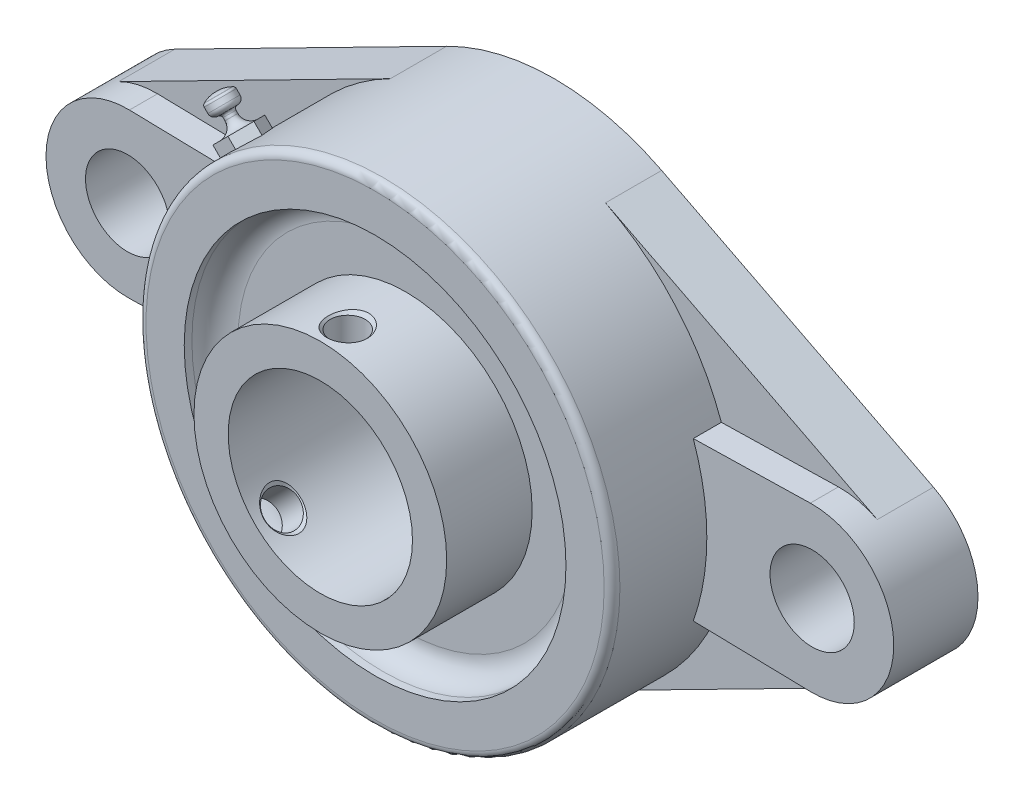
from build123d import *
from build123d.topology import SkipClean

# Parameters (mm, degrees)
SKETCH2_W          = 10.260420585
SKETCH2_H          = 10.310228453
CUT_EXTRUDE1_DEPTH = 4
SKETCH4_W          = 468
SKETCH4_H          = 360
CUT_EXTRUDE2_DEPTH = 44.4
SKETCH5_W          = 234
SKETCH5_H          = 180
CUT_EXTRUDE3_DEPTH = 5.333333333
SKETCH6_R          = 8
CUT_EXTRUDE4_DEPTH = 16
SKETCH7_R          = 8
CUT_EXTRUDE5_DEPTH = 16


with BuildPart() as part:
    # Sketch1 → Revolve1 (revolve)
    with BuildSketch(Plane(origin=(0, 0, 0), x_dir=(0, 0, -1), z_dir=(0.7071067811865476, 0.7071067811865475, 0)), mode=Mode.PRIVATE) as revolve1_sk:
        with BuildLine():
            Line((-4.44, 53), (-4.26179677, 53))
            ThreePointArc((-4.26179677, 53), (-3.226520589, 52.863703305), (-2.26179677, 52.464101615))
            Line((-2.26179677, 52.464101615), (-2.19, 52.422649731))
            ThreePointArc((-2.19, 52.422649731), (-2.006987298, 52.239637029), (-1.94, 51.989637029))
            Line((-1.94, 51.989637029), (-1.94, 51))
            ThreePointArc((-1.94, 51), (-2.232893219, 50.292893219), (-2.94, 50))
            ThreePointArc((-2.94, 50), (-3.293553391, 49.853553391), (-3.44, 49.5))
            Line((-3.44, 49.5), (-3.44, 49))
            ThreePointArc((-3.44, 49), (-2.854213562, 47.585786438), (-1.44, 47))
            Line((-1.44, 47), (0.56, 47))
            Line((0.56, 47), (0.56, 43))
            Line((0.56, 43), (-4.44, 43))
            Line((-4.44, 43), (-4.44, 53))
        make_face()
    revolve(revolve1_sk.sketch.rotate(Axis((-30.405591591, 30.405591591, 4.44), (-0.7071067811865477, 0.7071067811865474, 0)), 90), axis=Axis((-30.405591591, 30.405591591, 4.44), (-0.7071067811865477, 0.7071067811865474, 0)))

    # Sketch2 → Cut-Extrude1 (cut)
    with BuildSketch(Plane(origin=(-30.405591591, 30.405591591, 0), x_dir=(0, 0, -1), z_dir=(0.7071067811865501, -0.7071067811865449, 0))):
        with Locations((-4.564519667, -0.074711801)):
            Rectangle(SKETCH2_W, SKETCH2_H)
        Polygon((-7.94, 2.020725942), (-7.94, -2.020725942), (-4.44, -4.041451884), (-0.94, -2.020725942), (-0.94, 2.020725942), (-4.44, 4.041451884), align=None, mode=Mode.SUBTRACT)
    extrude(amount=-CUT_EXTRUDE1_DEPTH, mode=Mode.SUBTRACT)

    # Sketch3 → Revolve2 (revolve)
    with BuildSketch(Plane(origin=(0, 0, 0), x_dir=(0, 0, -1), z_dir=(1, 0, 0)), mode=Mode.PRIVATE) as revolve2_sk:
        with BuildLine():
            Line((-22.2, 24), (-22.2, 17.5))
            Line((-22.2, 17.5), (20.7, 17.5))
            Line((20.7, 17.5), (20.7, 24))
            Line((20.7, 24), (19.533333333, 24))
            ThreePointArc((19.533333333, 24), (15.408543776, 25.708543776), (13.7, 29.833333333))
            Line((13.7, 29.833333333), (13.7, 31.875))
            ThreePointArc((13.7, 31.875), (14.981407832, 34.968592168), (18.075, 36.25))
            Line((18.075, 36.25), (22.2, 36.25))
            Line((22.2, 36.25), (22.2, 80.5))
            Line((22.2, 80.5), (6.2, 80.5))
            Line((6.2, 80.5), (6.2, 45))
            Line((6.2, 45), (-10.3, 45))
            ThreePointArc((-10.3, 45), (-11.360660172, 44.560660172), (-11.8, 43.5))
            Line((-11.8, 43.5), (-11.8, 36.25))
            Line((-11.8, 36.25), (-10.341666667, 36.25))
            ThreePointArc((-10.341666667, 36.25), (-7.248074499, 34.968592168), (-5.966666667, 31.875))
            Line((-5.966666667, 31.875), (-5.966666667, 24))
            Line((-5.966666667, 24), (-22.2, 24))
        make_face()
    revolve(revolve2_sk.sketch.rotate(Axis((0, 0, -22.2), (0, 0, 1)), 270), axis=Axis((0, 0, -22.2), (0, 0, 1)))

    # Sketch4 → Cut-Extrude2 (cut)
    with SkipClean():  # the faces are left unmerged after this step: merging them gives an invalid solid
        with BuildSketch(Plane.XY):
            Rectangle(SKETCH4_W, SKETCH4_H)
            with BuildLine():
                Line((-72.034615385, -13.811740889), (-20.423076923, -40.098602582))
                ThreePointArc((-20.423076923, -40.098602582), (0, -45), (20.423076923, -40.098602582))
                Line((20.423076923, -40.098602582), (72.034615385, -13.811740889))
                ThreePointArc((72.034615385, -13.811740889), (80.5, 0), (72.034615385, 13.811740889))
                Line((72.034615385, 13.811740889), (20.423076923, 40.098602582))
                ThreePointArc((20.423076923, 40.098602582), (0, 45), (-20.423076923, 40.098602582))
                Line((-20.423076923, 40.098602582), (-72.034615385, 13.811740889))
                ThreePointArc((-72.034615385, 13.811740889), (-80.5, 0), (-72.034615385, -13.811740889))
            make_face(mode=Mode.SUBTRACT)
        extrude(amount=-CUT_EXTRUDE2_DEPTH, mode=Mode.SUBTRACT)

    # Sketch5 → Cut-Extrude3 (cut)
    with SkipClean():  # the faces are left unmerged after this step: merging them gives an invalid solid
        with BuildSketch(Plane.XY.offset(-6.2)):
            Rectangle(SKETCH5_W, SKETCH5_H)
            with BuildLine():
                Line((-64.654113716, -15.496140251), (-42.426406871, -15))
                ThreePointArc((-42.426406871, -15), (0, -45), (42.426406871, -15))
                Line((42.426406871, -15), (64.654113716, -15.496140251))
                ThreePointArc((64.654113716, -15.496140251), (80.5, 0), (64.654113716, 15.496140251))
                Line((64.654113716, 15.496140251), (42.426406871, 15))
                ThreePointArc((42.426406871, 15), (0, 45), (-42.426406871, 15))
                Line((-42.426406871, 15), (-64.654113716, 15.496140251))
                ThreePointArc((-64.654113716, 15.496140251), (-80.5, 0), (-64.654113716, -15.496140251))
            make_face(mode=Mode.SUBTRACT)
        extrude(amount=-CUT_EXTRUDE3_DEPTH, mode=Mode.SUBTRACT)

    # Sketch6 → Cut-Extrude4 (cut)
    with SkipClean():  # the faces are left unmerged after this step: merging them gives an invalid solid
        with BuildSketch(Plane.XY.offset(-6.2)):
            with Locations((-65, 0)):
                Circle(SKETCH6_R)
        extrude(amount=-CUT_EXTRUDE4_DEPTH, mode=Mode.SUBTRACT)

    # Sketch7 → Cut-Extrude5 (cut)
    with SkipClean():  # the faces are left unmerged after this step: merging them gives an invalid solid
        with BuildSketch(Plane.XY.offset(-6.2)):
            with Locations((65, 0)):
                Circle(SKETCH7_R)
        extrude(amount=-CUT_EXTRUDE5_DEPTH, mode=Mode.SUBTRACT)

    # Sketch8 → Cut-Revolve1 (revolve, cut)
    with SkipClean():  # the faces are left unmerged after this step: merging them gives an invalid solid
        with BuildSketch(Plane(origin=(0, 0, 0), x_dir=(0, 0, -1), z_dir=(1, 0, 0)), mode=Mode.PRIVATE) as cut_revolve1_sk:
            Polygon((-17, 24), (-13, 24), (-13.6765, 23.3235), (-13.6765, 17.6765), (-13, 17), (-17, 17), align=None)
        revolve(cut_revolve1_sk.sketch.rotate(Axis((0, 17, 17), (0, 1, 0)), 180), axis=Axis((0, 17, 17), (0, 1, 0)), mode=Mode.SUBTRACT)

    # Sketch9 → Cut-Revolve2 (revolve, cut)
    with SkipClean():  # the faces are left unmerged after this step: merging them gives an invalid solid
        with BuildSketch(Plane(origin=(0, 0, 0), x_dir=(0, 0, -1), z_dir=(0.7071067811865476, -0.7071067811865475, 0)), mode=Mode.PRIVATE) as cut_revolve2_sk:
            Polygon((-17, -17), (-13, -17), (-13.6765, -17.6765), (-13.6765, -23.3235), (-13, -24), (-17, -24), align=None)
        revolve(cut_revolve2_sk.sketch.rotate(Axis((-16.970562748, -16.970562748, 17), (0.7071067811865476, 0.7071067811865476, 0)), 90), axis=Axis((-16.970562748, -16.970562748, 17), (0.7071067811865476, 0.7071067811865476, 0)), mode=Mode.SUBTRACT)


solid = part.part
